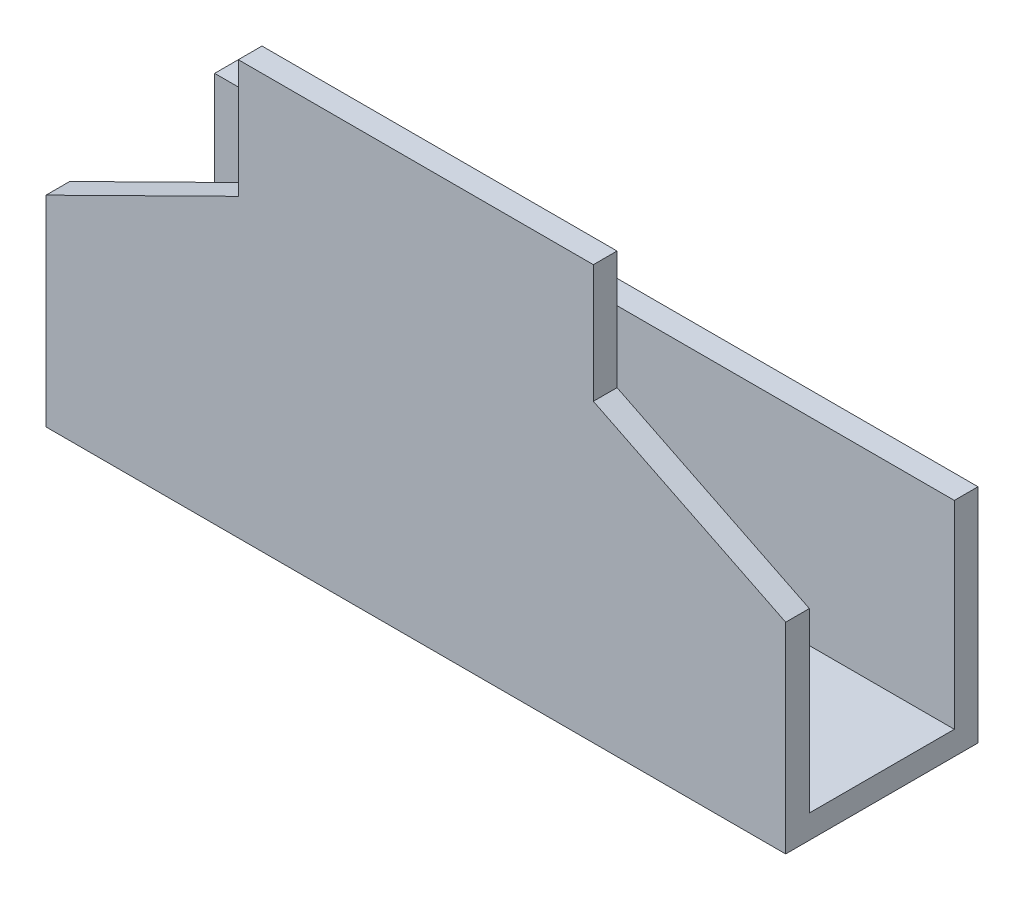
SolidWorks part; units mm, degrees
ref_plane "Front Plane" through (0, 0, 0) normal (0, 0, 1) x (1, 0, 0)
ref_plane "Top Plane" through (0, 0, 0) normal (0, 1, 0) x (1, 0, 0)
ref_plane "Right Plane" through (0, 0, 0) normal (1, 0, 0) x (0, 0, -1)
other "Configuration Table"
sketch "Sketch1" plane through (0, 0, 0) normal (0, 0, 1) x (1, 0, 0)
  line L0 (0, 0) -> (0, 280) construction
  line L1 (120, 280) -> (-120, 280)
  line L2 (-120, 280) -> (-120, 200)
  line L3 (-120, 200) -> (-250, 135.6978)
  line L4 (-250, 135.6978) -> (-250, 0)
  line L5 (-250, 0) -> (250, 0)
  line L6 (120, 200) -> (250, 135.6978)
  line L7 (120, 280) -> (120, 200)
  line L8 (250, 135.6978) -> (250, 0)
  dimension "D1" = 280
  dimension "D2" = 120
  dimension "D3" = 80
  dimension "D4" = 250
extrude "Boss-Extrude1" add sketch "Sketch1" along normal blind 16
sketch "Sketch2" plane through (0, 0, 16) normal (0, 0, 1) x (1, 0, 0)
  line L1 (-250, 16) -> (250, 16)
  line L2 (-250, 16) -> (-250, 0)
  line L3 (-250, 0) -> (250, 0)
  line L4 (250, 16) -> (250, 0)
  line L5 (-250, 16) -> (250, 0) construction
  line L6 (-250, 0) -> (250, 16) construction
  point P0 (0, 8)
  dimension "D1" = 16
extrude "Boss-Extrude2" add sketch "Sketch2" against normal blind 130
sketch "Sketch3" plane through (0, 0, 0) normal (0, -1, 0) x (-1, 0, 0)
  line L0 (250, -16) -> (250, 114) construction
  line L1 (250, 98) -> (-250, 98)
  line L2 (250, 98) -> (250, 114)
  line L3 (250, 114) -> (-250, 114)
  line L4 (-250, 98) -> (-250, 114)
  line L5 (250, 98) -> (-250, 114) construction
  line L6 (250, 114) -> (-250, 98) construction
  point P0 (0, 106)
  dimension "D1" = 16
extrude "Boss-Extrude3" add sketch "Sketch3" against normal blind 150
